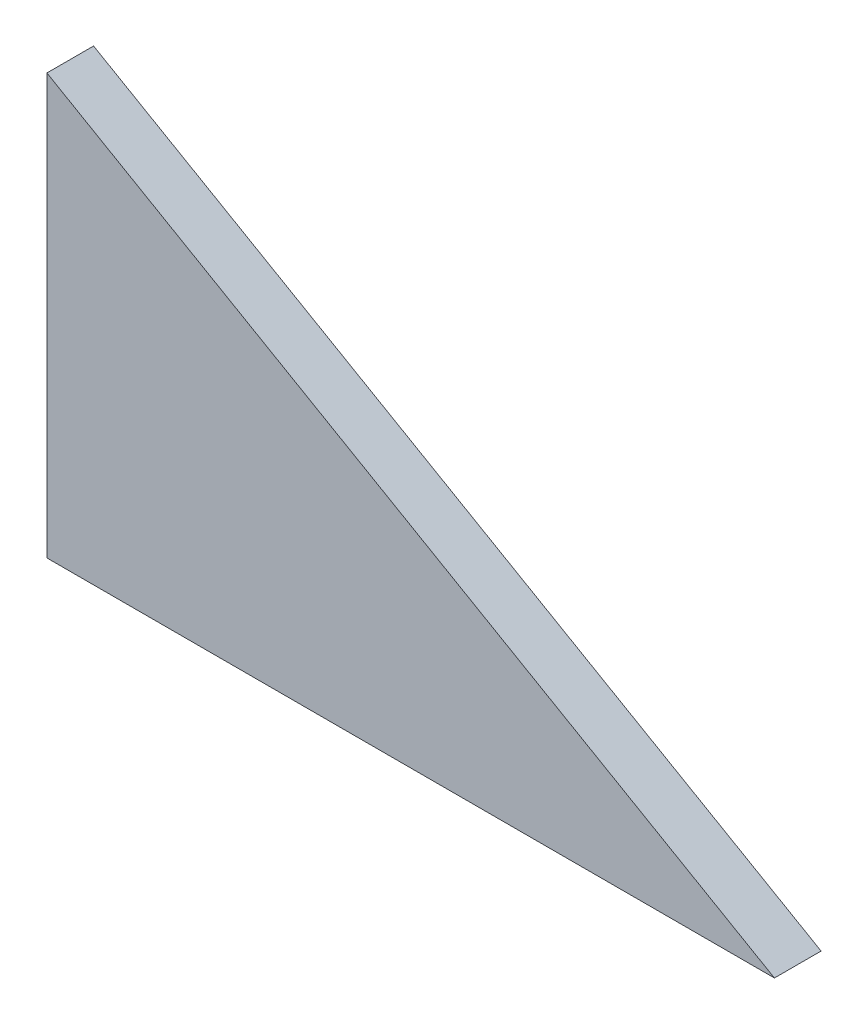
SolidWorks part; units mm, degrees
ref_plane "Front Plane" through (0, 0, 0) normal (0, 0, 1) x (1, 0, 0)
ref_plane "Top Plane" through (0, 0, 0) normal (0, 1, 0) x (1, 0, 0)
ref_plane "Right Plane" through (0, 0, 0) normal (1, 0, 0) x (0, 0, -1)
sketch "Sketch1" plane through (0, 0, 0) normal (0, 0, 1) x (1, 0, 0)
  line L0 (0, 0) -> (0, -90)
  line L1 (0, -90) -> (155.8846, -90)
  line L2 (155.8846, -90) -> (0, 0)
  dimension "D1" = 90
  dimension "D2" = 30
extrude "Boss-Extrude1" add sketch "Sketch1" along normal blind 10
